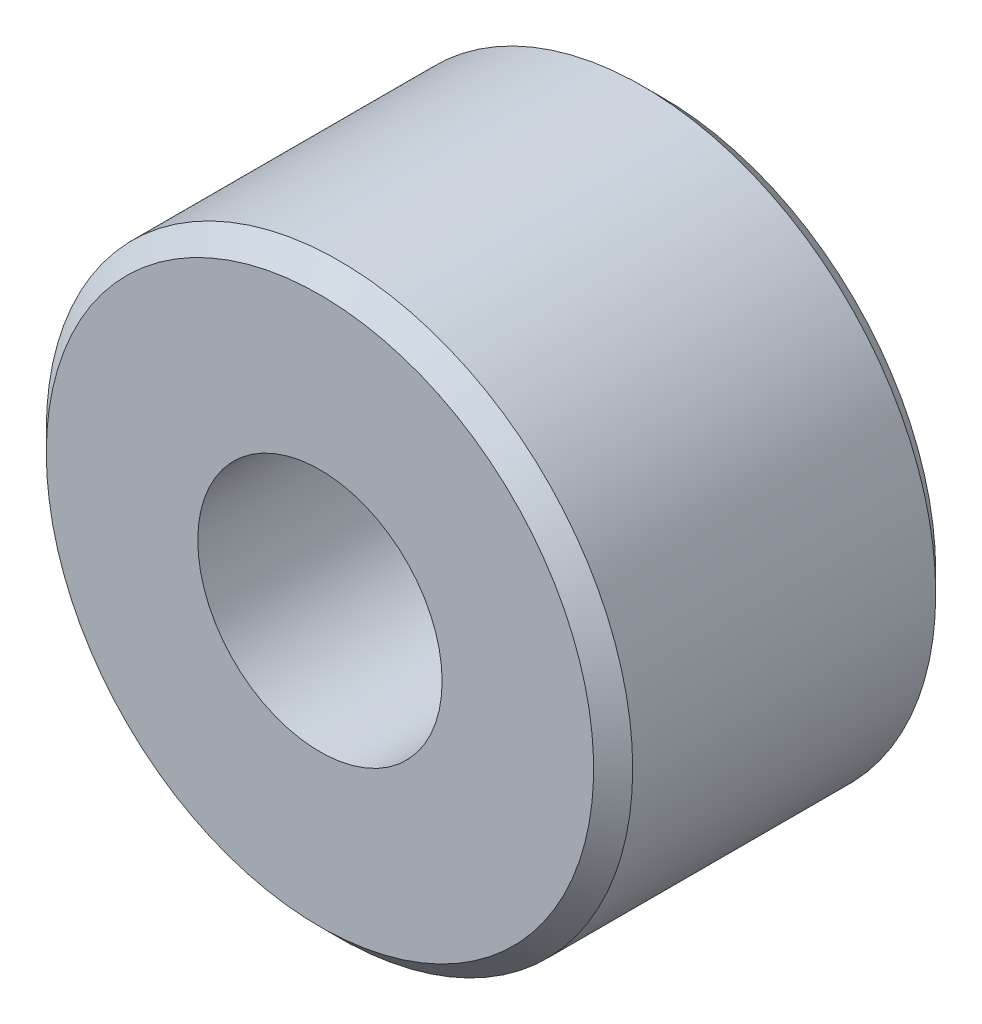
from build123d import *

# Parameters (mm, degrees)
SKETCH1_R             = 3
BOSS_EXTRUDE1_DEPTH   = 3.5
M3_TAPPED_HOLE1_D     = 2.5
M3_TAPPED_HOLE1_DEPTH = 7.5
CHAMFER1_SIZE         = 0.2


with BuildPart() as part:
    # Sketch1 → Boss-Extrude1 (new body)
    with BuildSketch(Plane.XY):
        Circle(SKETCH1_R)
    extrude(amount=BOSS_EXTRUDE1_DEPTH)

    # M3 Tapped Hole1
    with Locations(Plane(origin=(0, 0, 0), x_dir=(-1, 0, 0), z_dir=(0, 0, -1))):
        with Locations((0, 0)):
            Hole(M3_TAPPED_HOLE1_D / 2, depth=M3_TAPPED_HOLE1_DEPTH)

    # Chamfer1
    chamfer1_edges = [part.edges().sort_by_distance(p)[0] for p in [
        (-3, 0, 0),
        (-3, 0, 3.5),
    ]]
    chamfer(chamfer1_edges, length=CHAMFER1_SIZE)


solid = part.part
